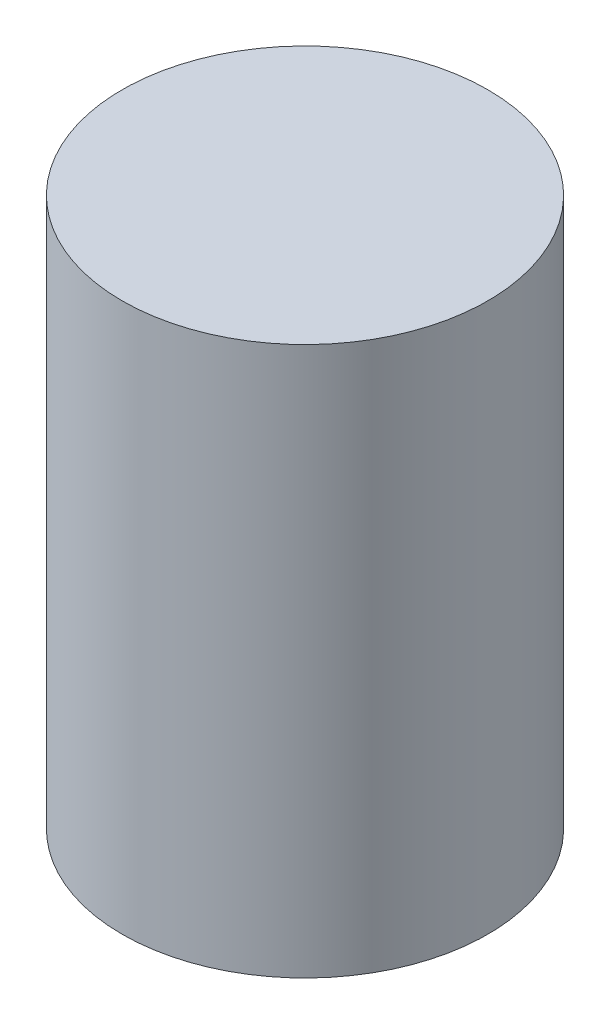
from build123d import *

# Parameters (mm, degrees)
SKETCH1_R           = 10
BOSS_EXTRUDE1_DEPTH = 30


with BuildPart() as part:
    # Sketch1 → Boss-Extrude1 (new body)
    with BuildSketch(Plane(origin=(0, 0, 0), x_dir=(1, 0, 0), z_dir=(0, 1, 0))):
        with Locations(Location((0, 0, 0), (0, 0, 270))):
            Circle(SKETCH1_R)
    extrude(amount=BOSS_EXTRUDE1_DEPTH)


solid = part.part
